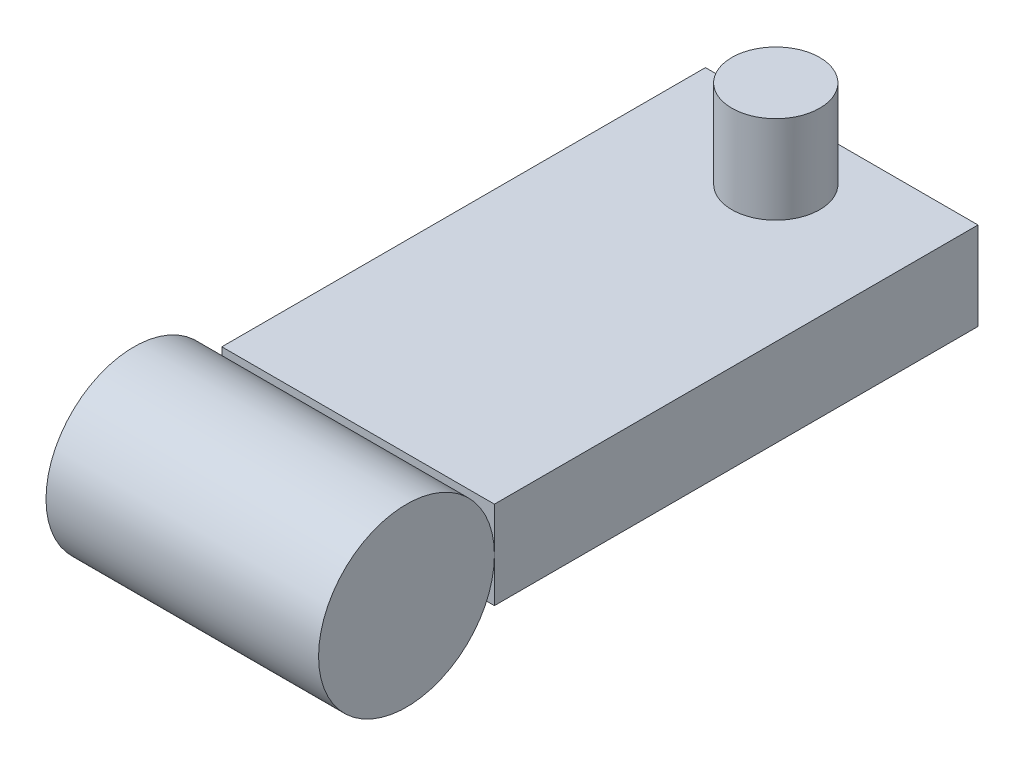
from build123d import *

# Parameters (mm, degrees)
SKETCH_1_W      = 62
SKETCH_1_H      = 20
EXTRUDE_1_DEPTH = 110
SKETCH_2_R      = 20
EXTRUDE_2_DEPTH = 62
SKETCH_3_R      = 10
EXTRUDE_3_DEPTH = 20


with BuildPart() as part:
    # 草图1 → 凸台-拉伸1 (new body)
    with BuildSketch(Plane.XY):
        Rectangle(SKETCH_1_W, SKETCH_1_H)
    extrude(amount=EXTRUDE_1_DEPTH)

    # 草图3 → 凸台-拉伸3 (add)
    with BuildSketch(Plane(origin=(0, 10, 0), x_dir=(1, 0, 0), z_dir=(0, 1, 0))):
        with Locations(Location((0, -15, 0), (0, 0, 90))):
            Circle(SKETCH_3_R)
    extrude(amount=EXTRUDE_3_DEPTH)


with BuildPart() as body_2:
    # 草图2 → 凸台-拉伸2 (new body)
    with BuildSketch(Plane(origin=(31, 0, 0), x_dir=(0, 0, -1), z_dir=(1, 0, 0))):
        with Locations((-130, 0)):
            Circle(SKETCH_2_R)
    extrude(amount=-EXTRUDE_2_DEPTH)


solid = Compound([part.part, body_2.part])
